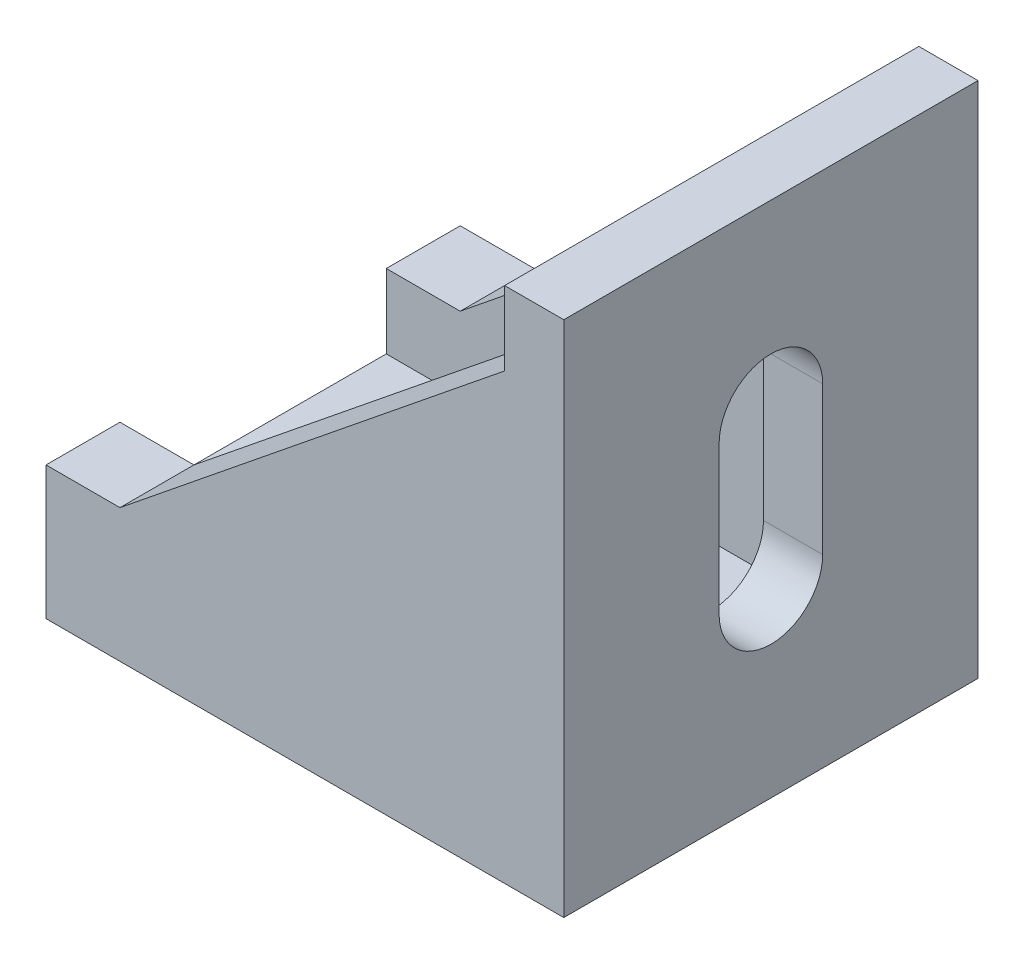
SolidWorks part; units mm, degrees
ref_plane "前视基准面" through (0, 0, 0) normal (0, 0, 1) x (1, 0, 0)
ref_plane "上视基准面" through (0, 0, 0) normal (0, 1, 0) x (1, 0, 0)
ref_plane "右视基准面" through (0, 0, 0) normal (1, 0, 0) x (0, 0, -1)
sketch "草图1" plane through (0, 0, 0) normal (0, 0, 1) x (1, 0, 0)
  line L1 (2, -17.5) -> (-2, -17.5)
  line L2 (2, -17.5) -> (2, 17.5)
  line L3 (2, 17.5) -> (-2, 17.5)
  line L4 (-2, -17.5) -> (-2, 17.5)
  line L5 (2, -17.5) -> (-2, 17.5) construction
  line L6 (2, 17.5) -> (-2, -17.5) construction
  line L7 (-33, -13.5) -> (2, -13.5)
  line L8 (-33, -13.5) -> (-33, -17.5)
  line L9 (-33, -17.5) -> (2, -17.5)
  line L10 (2, -13.5) -> (2, -17.5)
  line L11 (-33, -13.5) -> (2, -17.5) construction
  line L12 (-33, -17.5) -> (2, -13.5) construction
  point P0 (0, 0)
  point P5 (-15.5, -15.5)
  dimension "D1" = 4
  dimension "D2" = 35
extrude "凸台-拉伸1" add sketch "草图1" along normal mid plane 28 contours L4 L7 L2 L3 | L7 L4 L1 L2 | L8 L9 L4 L7
sketch "草图2" plane through (0, 0, -14) normal (0, 0, -1) x (-1, 0, 0)
  line L0 (2, 12.5) -> (28, -8.5)
  line L1 (2, -13.5) -> (2, 17.5) construction
  line L2 (28, -8.5) -> (33, -8.5)
  line L3 (33, -8.5) -> (33, -13.5)
  line L4 (33, -13.5) -> (2, -13.5)
  line L5 (33, -13.5) -> (2, -13.5) construction
  line L7 (2, -13.5) -> (2, 12.5)
  line L8 (-2, 17.5) -> (2, 17.5) construction
  dimension "D1" = 5
  dimension "D2" = 5
  dimension "D3" = 5
extrude "凸台-拉伸2" add sketch "草图2" against normal blind 5
mirror "镜向1" about plane through (0, 0, 0) normal (0, 0, 1) of "凸台-拉伸2"
sketch "草图3" plane through (-2, 0, 0) normal (-1, 0, 0) x (0, 0, 1)
  line L0 (0, -5) -> (0, 5) construction
  line L1 (-3.5, -5) -> (-3.5, 5)
  line L2 (3.5, -5) -> (3.5, 5)
  arc A0 (-3.5, -5) -> (3.5, -5) centre (0, -5) ccw
  arc A1 (3.5, 5) -> (-3.5, 5) centre (0, 5) ccw
  point P2 (0, 0)
  dimension "D2" = 10
  dimension "D1" = 7
extrude "切除-拉伸1" cut sketch "草图3" against normal blind 5
sketch "草图4" plane through (0, -13.5, 0) normal (0, 1, 0) x (1, 0, 0)
  line L0 (-15, 14) -> (-15, -14) construction
  line L1 (-28, 14) -> (-2, 14) construction
  line L2 (-28, -14) -> (-2, -14) construction
  line L3 (-20, 0) -> (-10, 0) construction
  line L4 (-20, 3.5) -> (-10, 3.5)
  line L5 (-20, -3.5) -> (-10, -3.5)
  arc A0 (-20, 3.5) -> (-20, -3.5) centre (-20, 0) ccw
  arc A1 (-10, -3.5) -> (-10, 3.5) centre (-10, 0) ccw
  point P8 (-15, 0)
  dimension "D1" = 7
  dimension "D2" = 10
extrude "切除-拉伸2" cut sketch "草图4" against normal blind 5
